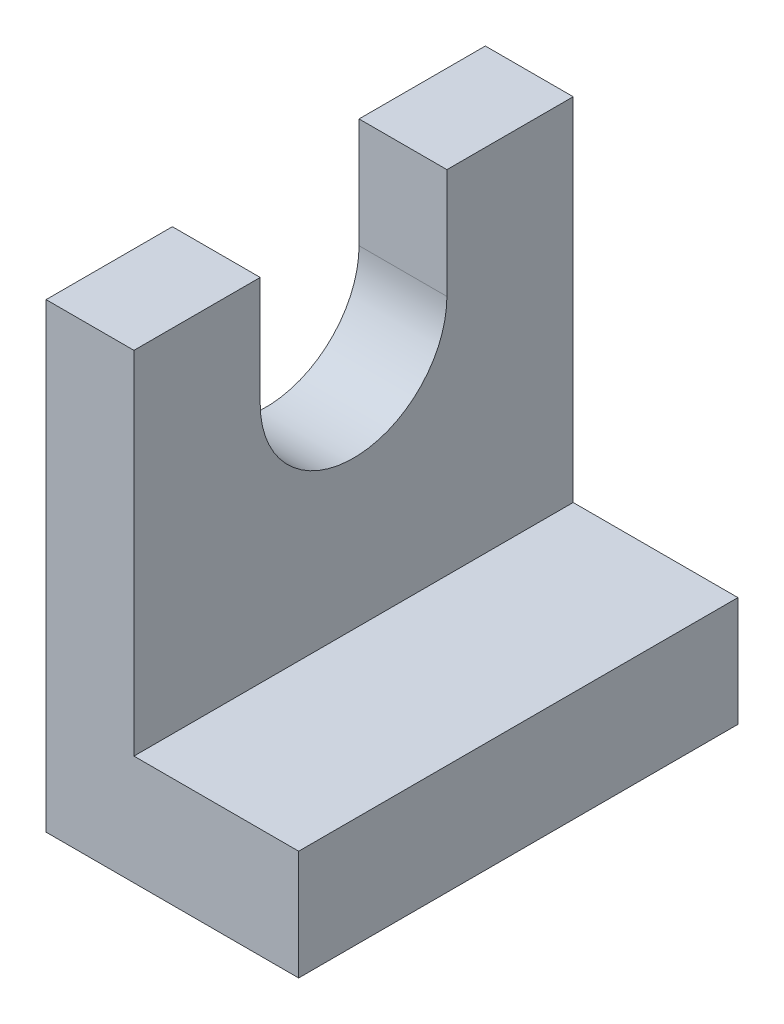
from build123d import *

# Parameters (mm, degrees)
EXTRUDE_1_DEPTH     = 20
CUT_EXTRUDE_1_REACH = 50.877


with BuildPart() as part:
    # 草图1 → 凸台-拉伸1 (new, symmetric)
    with BuildSketch(Plane.XY):
        Polygon((0, 0), (23, 0), (23, 10), (8, 10), (8, 42), (0, 42), align=None)
    extrude(amount=EXTRUDE_1_DEPTH, both=True)

    # 草图2 → 切除-拉伸1 (cut, up to next)
    with BuildSketch(Plane(origin=(8, 0, 0), x_dir=(0, 0, -1), z_dir=(1, 0, 0)), mode=Mode.PRIVATE) as cut_extrude_1_sk1:
        with BuildLine():
            Line((-8.5, 42), (-8.5, 32))
            ThreePointArc((-8.5, 32), (0, 23.5), (8.5, 32))
            Line((8.5, 32), (8.5, 42))
            Line((8.5, 42), (-8.5, 42))
        make_face()
    cut_extrude_1_tool1 = extrude(cut_extrude_1_sk1.sketch, amount=-CUT_EXTRUDE_1_REACH, mode=Mode.PRIVATE) & part.part
    add(cut_extrude_1_tool1.solids().sort_by_distance((8, 33.55414, 0))[0], mode=Mode.SUBTRACT)


solid = part.part
